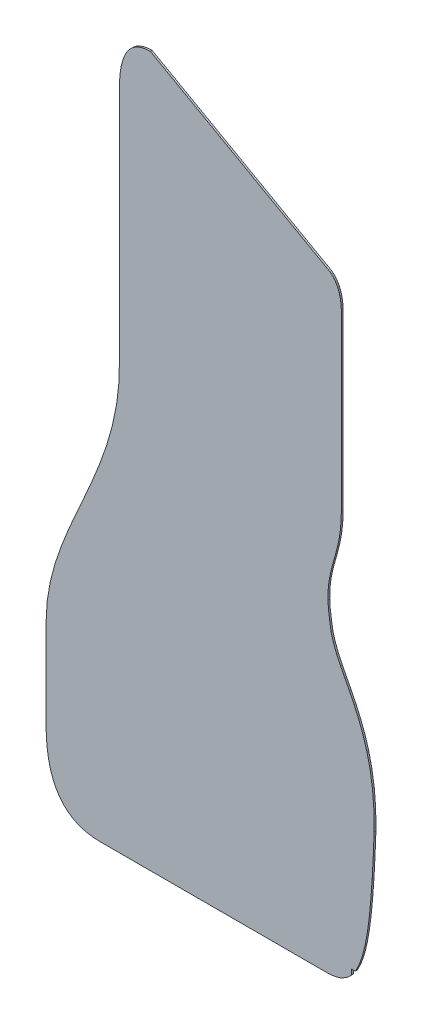
from build123d import *

# Parameters (mm, degrees)
EXTRUDE_1_DEPTH     = 1.5
SKETCH_2_W          = 32
SKETCH_2_H          = 22
CUT_EXTRUDE_1_DEPTH = 10


with BuildPart() as part:
    # 草图1 → 凸台-拉伸1 (new, symmetric)
    with BuildSketch(Plane.XY):
        Polygon((103, 235), (-24.833333333, 235), (-152.666666667, 235), (-280.5, 235), (-293.035714286, 235.637755102), (-304.642857143, 237.551020408), (-315.321428571, 240.739795918), (-325.071428571, 245.204081633), (-333.892857143, 250.943877551), (-341.785714286, 257.959183673), (-348.75, 266.25), (-354.785714286, 275.816326531), (-359.892857143, 286.658163265), (-364.071428571, 298.775510204), (-367.321428571, 312.168367347), (-369.642857143, 326.836734694), (-371.035714286, 342.780612245), (-371.5, 360), (-371.5, 410), (-371.5, 460), (-371.5, 510), (-369.607325073, 541.716472303), (-364.317784257, 572.711370262), (-356.214103499, 603.18148688), (-345.879008746, 633.32361516), (-333.895225948, 663.334548105), (-320.84548105, 693.411078717), (-307.3125, 723.75), (-293.879008746, 754.548104956), (-281.127733236, 786.002186589), (-269.641399417, 818.309037901), (-260.002733236, 851.665451895), (-252.794460641, 886.268221574), (-248.59930758, 922.314139942), (-248, 960), (-248, 1090), (-248, 1220), (-248, 1350), (-247.734693878, 1361.020408163), (-246.93877551, 1371.224489796), (-245.612244898, 1380.612244898), (-243.755102041, 1389.183673469), (-241.367346939, 1396.93877551), (-238.448979592, 1403.87755102), (-235, 1410), (-231.020408163, 1415.306122449), (-226.510204082, 1419.795918367), (-221.469387755, 1423.469387755), (-215.897959184, 1426.326530612), (-209.795918367, 1428.367346939), (-203.163265306, 1429.591836735), (-196, 1430), (-95.25, 1373.333333333), (5.5, 1316.666666667), (106.25, 1260), (108.93622449, 1257.887755102), (111.423469388, 1255.551020408), (113.711734694, 1252.989795918), (115.801020408, 1250.204081633), (117.691326531, 1247.193877551), (119.382653061, 1243.959183673), (120.875, 1240.5), (122.168367347, 1236.816326531), (123.262755102, 1232.908163265), (124.158163265, 1228.775510204), (124.854591837, 1224.418367347), (125.352040816, 1219.836734694), (125.650510204, 1215.030612245), (125.75, 1210), (125.75, 1113.333333333), (125.75, 1016.666666667), (125.75, 920), (125.280976676, 904.7303207), (123.987609329, 890.903790087), (122.040451895, 878.279883382), (119.610058309, 866.618075802), (116.866982507, 855.677842566), (113.981778426, 845.218658892), (111.125, 835), (108.467201166, 824.781341108), (106.17893586, 814.322157434), (104.430758017, 803.381924198), (103.393221574, 791.720116618), (103.236880466, 779.096209913), (104.13228863, 765.2696793), (106.25, 750), (108.586825802, 735.40451895), (112.60787172, 721.39941691), (118.007561953, 707.656705539), (124.4803207, 693.848396501), (131.720572157, 679.646501458), (139.422740525, 664.72303207), (147.28125, 648.75), (154.990524781, 631.39941691), (162.244989067, 612.343294461), (168.739067055, 591.253644315), (174.167182945, 567.802478134), (178.223760933, 541.66180758), (180.603225219, 512.503644315), (181, 480), (179.493440233, 443.170553936), (177.702623907, 409.752186589), (175.542274052, 379.635568513), (172.927113703, 352.711370262), (169.771865889, 328.870262391), (165.991253644, 308.002915452), (161.5, 290), (156.212827988, 274.752186589), (150.044460641, 262.150145773), (142.909620991, 252.084548105), (134.72303207, 244.44606414), (125.39941691, 239.125364431), (114.853498542, 236.013119534), align=None)
    extrude(amount=EXTRUDE_1_DEPTH, both=True)

    # 草图2 → 切除-拉伸1 (cut, symmetric)
    with BuildSketch(Plane.XY):
        with Locations((159, 250)):
            Rectangle(SKETCH_2_W, SKETCH_2_H)
        with Locations((159, 1150)):
            Rectangle(SKETCH_2_W, SKETCH_2_H)
    extrude(amount=CUT_EXTRUDE_1_DEPTH, both=True, mode=Mode.SUBTRACT)


solid = part.part
